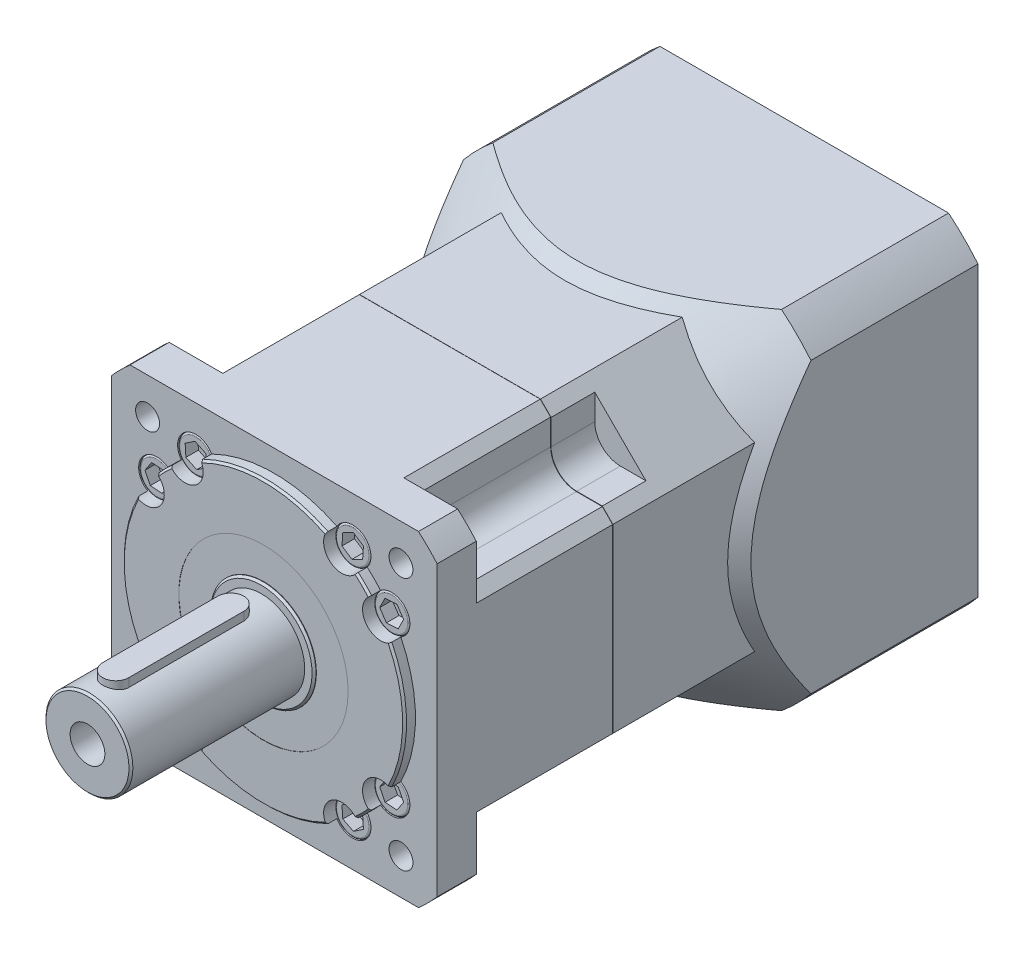
from build123d import *
from build123d.topology import SkipClean

# Parameters (mm, degrees)
EXTRUDE_START                    = 8
EXTRUDE_2_DEPTH                  = 15
CHAMFER_1_SIZE                   = 0.9
EXTRUDE_START_2                  = 49.5
SKETCH_6_W                       = 150
SKETCH_6_H                       = 150
EXTRUDE_1_DEPTH                  = 194.5
SKETCH_7_R                       = 5.5
CUT_EXTRUDE_1_DEPTH              = 18
CUT_EXTRUDE_START                = 226
CUT_EXTRUDE_3_DEPTH              = 176.5
CUT_EXTRUDE_2_DEPTH              = 83
CUT_EXTRUDE_4_DEPTH              = 62.8
PATTERN_CIRCULAR_1_COUNT         = 4
SKETCH_11_R                      = 8.4
CUT_EXTRUDE_5_DEPTH              = 5
CUT_EXTRUDE_START_2              = 244
SKETCH_12_R                      = 8.4
SKETCH_12_R_2                    = 8.25
CUT_EXTRUDE_6_DEPTH              = 9.9
CUT_EXTRUDE_7_DEPTH              = 5.775
FILLET_1_R                       = 0.825
PATTERN_CIRCULAR_2_COUNT         = 16
FILLET_1_OF_PATTERN_CIRCULAR_2_R = 0.825
CUT_EXTRUDE_START_3              = 248.9
SKETCH_14_R                      = 39
SKETCH_14_R_2                    = 24.3
CUT_EXTRUDE_8_DEPTH              = 0.1
EXTRUDE_3_DEPTH                  = 49.5
SKETCH_17_R                      = 4
CUT_EXTRUDE_9_DEPTH              = 24
PATTERN_CIRCULAR_3_COUNT         = 4
SKETCH_27_R                      = 150
CUT_EXTRUDE_15_DEPTH             = 143
SKETCH_21_R                      = 6.15
CUT_EXTRUDE_10_DEPTH             = 10
CUT_EXTRUDE_START_4              = 10
SKETCH_22_R                      = 6.15
SKETCH_22_R_2                    = 6
CUT_EXTRUDE_12_DEPTH             = 7.2
CUT_EXTRUDE_13_DEPTH             = 4.2
FILLET_2_R                       = 0.6
PATTERN_CIRCULAR_4_COUNT         = 4
FILLET_2_OF_PATTERN_CIRCULAR_4_R = 0.6
EXTRUDE_START_3                  = 10
EXTRUDE_4_DEPTH                  = 1
SKETCH_25_W                      = 150
SKETCH_25_H                      = 0.1
CUT_EXTRUDE_14_DEPTH             = 150


with BuildPart() as part:
    # 草图4 → 旋转1 (revolve)
    with BuildSketch(Plane(origin=(0, 0, 0), x_dir=(0, 0, -1), z_dir=(1, 0, 0))):
        Polygon((-249, 65), (-244, 65), (-244, 0), (-305.381197846, 0), (-310, 8), (-330, 8), (-330, 20), (-250, 20), (-250, 24.3), (-249, 24.3), align=None)
    revolve(axis=Axis((0, 0, 244), (0, 0, 1)))

    # 草图15 → 凸台-拉伸2 (add)
    with BuildSketch(Plane(origin=(0, 0, 0), x_dir=(1, 0, 0), z_dir=(0, 1, 0)).offset(EXTRUDE_START)):
        with BuildLine():
            Line((-6, -317), (-6, -264))
            ThreePointArc((-6, -264), (0, -258), (6, -264))
            Line((6, -264), (6, -317))
            ThreePointArc((6, -317), (0, -323), (-6, -317))
        make_face()
    extrude(amount=EXTRUDE_2_DEPTH)

    # 倒角1
    chamfer_1_edges = [part.edges().sort_by_distance(p)[0] for p in [
        (0, -65, 249),
        (0, -24.3, 250),
        (0, -20, 330),
    ]]
    chamfer(chamfer_1_edges, length=CHAMFER_1_SIZE)

    # 草图6 → 凸台-拉伸1 (add)
    with BuildSketch(Plane.XY.offset(EXTRUDE_START_2)):
        Rectangle(SKETCH_6_W, SKETCH_6_H)
    extrude(amount=EXTRUDE_1_DEPTH)

    # 草图7 → 切除-拉伸1 (cut)
    with BuildSketch(Plane.XY.offset(244)):
        with Locations((58.336309448, 58.336309448)):
            Circle(SKETCH_7_R)
        with BuildLine():
            Line((66.40732664, 75), (75, 75))
            Line((75, 75), (75, 66.40732664))
            ThreePointArc((75, 66.40732664), (70.834077362, 70.834077362), (66.40732664, 75))
        make_face()
    cut_extrude_1 = extrude(amount=-CUT_EXTRUDE_1_DEPTH, mode=Mode.SUBTRACT)

    # 草图9 → 切除-拉伸3 (cut)
    with BuildSketch(Plane.XY.offset(CUT_EXTRUDE_START)):
        Polygon((41.672618896, 75), (75, 41.672618896), (75, 75), align=None)
    cut_extrude_3 = extrude(amount=-CUT_EXTRUDE_3_DEPTH, mode=Mode.SUBTRACT)

    # 草图8 → 切除-拉伸2 (cut)
    with BuildSketch(Plane.XY.offset(CUT_EXTRUDE_START)):
        with BuildLine():
            Line((58.336309448, 46.553300859), (75, 46.553300859))
            Line((75, 46.553300859), (75, 75))
            Line((75, 75), (46.553300859, 75))
            Line((46.553300859, 75), (46.553300859, 58.336309448))
            ThreePointArc((46.553300859, 58.336309448), (50.004464172, 50.004464172), (58.336309448, 46.553300859))
        make_face()
    cut_extrude_2 = extrude(amount=-CUT_EXTRUDE_2_DEPTH, mode=Mode.SUBTRACT)

    # 草图10 → 切除-拉伸4 (cut)
    with BuildSketch(Plane(origin=(0, 0, 226), x_dir=(-1, 0, 0), z_dir=(0, 0, -1))):
        with BuildLine():
            Line((-46.553300859, 70.119318037), (-46.553300859, 58.336309448))
            ThreePointArc((-46.553300859, 58.336309448), (-50.004464172, 50.004464172), (-58.336309448, 46.553300859))
            Line((-58.336309448, 46.553300859), (-70.119318037, 46.553300859))
            Line((-70.119318037, 46.553300859), (-70.219318037, 46.453300859))
            Line((-70.219318037, 46.453300859), (-58.336309448, 46.453300859))
            ThreePointArc((-58.336309448, 46.453300859), (-49.933753494, 49.933753494), (-46.453300859, 58.336309448))
            Line((-46.453300859, 58.336309448), (-46.453300859, 70.219318037))
            Line((-46.453300859, 70.219318037), (-46.553300859, 70.119318037))
        make_face()
    cut_extrude_4 = extrude(amount=CUT_EXTRUDE_4_DEPTH, mode=Mode.SUBTRACT)

    # 阵列(圆周)1: 切除-拉伸1, 切除-拉伸3, 切除-拉伸2, 切除-拉伸4 ×4 about axis
    pattern_circular_1_axis = Axis((0, 0, 0), (0, 0, 1))
    add([cut_extrude_1.rotate(pattern_circular_1_axis, i * 360 / PATTERN_CIRCULAR_1_COUNT) for i in range(1, PATTERN_CIRCULAR_1_COUNT)], mode=Mode.SUBTRACT)
    add([cut_extrude_3.rotate(pattern_circular_1_axis, i * 360 / PATTERN_CIRCULAR_1_COUNT) for i in range(1, PATTERN_CIRCULAR_1_COUNT)], mode=Mode.SUBTRACT)
    add([cut_extrude_2.rotate(pattern_circular_1_axis, i * 360 / PATTERN_CIRCULAR_1_COUNT) for i in range(1, PATTERN_CIRCULAR_1_COUNT)], mode=Mode.SUBTRACT)
    add([cut_extrude_4.rotate(pattern_circular_1_axis, i * 360 / PATTERN_CIRCULAR_1_COUNT) for i in range(1, PATTERN_CIRCULAR_1_COUNT)], mode=Mode.SUBTRACT)

    # 草图11 → 切除-拉伸5 (cut)
    with BuildSketch(Plane.XY.offset(249)):
        with Locations((36.112065146, 54.0455248)):
            Circle(SKETCH_11_R)
    cut_extrude_5 = extrude(amount=-CUT_EXTRUDE_5_DEPTH, mode=Mode.SUBTRACT)

    # 草图12 → 切除-拉伸6 (cut)
    with BuildSketch(Plane.XY.offset(CUT_EXTRUDE_START_2)):
        with Locations((36.112065146, 54.0455248)):
            Circle(SKETCH_12_R)
        with Locations((36.112065146, 54.0455248)):
            Circle(SKETCH_12_R_2, mode=Mode.SUBTRACT)
    cut_extrude_6 = extrude(amount=-CUT_EXTRUDE_6_DEPTH, mode=Mode.SUBTRACT)

    # 草图13 → 切除-拉伸7 (cut)
    with BuildSketch(Plane.XY.offset(CUT_EXTRUDE_START_2)):
        Polygon((40.685148014, 50.989888518), (41.044865225, 56.478112596), (36.471782357, 59.533748877), (31.538982279, 57.101161081), (31.179265068, 51.612937003), (35.752347936, 48.557300722), align=None)
    cut_extrude_7 = extrude(amount=-CUT_EXTRUDE_7_DEPTH, mode=Mode.SUBTRACT)

    # 圆角1
    fillet_1_edges = [part.edges().sort_by_distance(p)[0] for p in [
        (27.862065146, 54.0455248, 244),
    ]]
    fillet(fillet_1_edges, radius=FILLET_1_R)

    # 阵列(圆周)2: 切除-拉伸5, 切除-拉伸6, 切除-拉伸7 ×16 about axis, 8 skipped
    pattern_circular_2_axis = Axis((0, 0, 0), (0, 0, -1))
    add([cut_extrude_5.rotate(pattern_circular_2_axis, i * 360 / PATTERN_CIRCULAR_2_COUNT) for i in range(1, PATTERN_CIRCULAR_2_COUNT) if i not in (2, 3, 6, 7, 10, 11, 14, 15)], mode=Mode.SUBTRACT)
    add([cut_extrude_6.rotate(pattern_circular_2_axis, i * 360 / PATTERN_CIRCULAR_2_COUNT) for i in range(1, PATTERN_CIRCULAR_2_COUNT) if i not in (2, 3, 6, 7, 10, 11, 14, 15)], mode=Mode.SUBTRACT)
    add([cut_extrude_7.rotate(pattern_circular_2_axis, i * 360 / PATTERN_CIRCULAR_2_COUNT) for i in range(1, PATTERN_CIRCULAR_2_COUNT) if i not in (2, 3, 6, 7, 10, 11, 14, 15)], mode=Mode.SUBTRACT)

    # 圆角1 of 阵列(圆周)2
    fillet_1_of_pattern_circular_2_edges = [part.edges().sort_by_distance(p)[0] for p in [
        (46.423518656, 39.269203463, 244),
        (54.0455248, -27.862065146, 244),
        (39.269203463, -46.423518656, 244),
        (-27.862065146, -54.0455248, 244),
        (-46.423518656, -39.269203463, 244),
        (-54.0455248, 27.862065146, 244),
        (-39.269203463, 46.423518656, 244),
    ]]
    fillet(fillet_1_of_pattern_circular_2_edges, radius=FILLET_1_OF_PATTERN_CIRCULAR_2_R)

    # 草图14 → 切除-拉伸8 (cut)
    with BuildSketch(Plane.XY.offset(CUT_EXTRUDE_START_3)):
        Circle(SKETCH_14_R)
        with Locations(Location((0, 0, 0), (0, 0, 90))):
            Circle(SKETCH_14_R_2, mode=Mode.SUBTRACT)
    extrude(amount=CUT_EXTRUDE_8_DEPTH, mode=Mode.SUBTRACT)

    # 草图16 → 凸台-拉伸3 (add)
    with BuildSketch(Plane.XY):
        with BuildLine():
            Line((80, -66.452990903), (80, 66.452990903))
            ThreePointArc((80, 66.452990903), (73.539105243, 73.539105243), (66.452990903, 80))
            Line((66.452990903, 80), (-66.452990903, 80))
            ThreePointArc((-66.452990903, 80), (-73.539105243, 73.539105243), (-80, 66.452990903))
            Line((-80, 66.452990903), (-80, -66.452990903))
            ThreePointArc((-80, -66.452990903), (-73.539105243, -73.539105243), (-66.452990903, -80))
            Line((-66.452990903, -80), (66.452990903, -80))
            ThreePointArc((66.452990903, -80), (73.539105243, -73.539105243), (80, -66.452990903))
        make_face()
    extrude(amount=EXTRUDE_3_DEPTH)

    # 草图17 → 切除-拉伸9 (cut)
    with BuildSketch(Plane.XY):
        with Locations((51.265241636, 51.265241636)):
            Circle(SKETCH_17_R)
    cut_extrude_9 = extrude(amount=CUT_EXTRUDE_9_DEPTH, mode=Mode.SUBTRACT)

    # 阵列(圆周)3: 切除-拉伸9 ×4 about axis
    pattern_circular_3_axis = Axis((0, 0, 0), (0, 0, 1))
    for i in range(1, PATTERN_CIRCULAR_3_COUNT):
        add(cut_extrude_9.rotate(pattern_circular_3_axis, i * 360 / PATTERN_CIRCULAR_3_COUNT), mode=Mode.SUBTRACT)

    # 草图26 → 旋转2 (revolve)
    with BuildSketch(Plane(origin=(0, 0, 0), x_dir=(0, 0, -1), z_dir=(1, 0, 0)), mode=Mode.PRIVATE) as revolve_2_sk:
        Polygon((-24, 150), (-24, 0), (-196.552629984, 0), align=None)
    revolve(revolve_2_sk.sketch.rotate(Axis((0, 0, 196.552629984), (0, 0, -1)), 180), axis=Axis((0, 0, 196.552629984), (0, 0, -1)))

    # 草图27 → 切除-拉伸15 (cut)
    with BuildSketch(Plane(origin=(0, 0, 0), x_dir=(-1, 0, 0), z_dir=(0, 0, -1))):
        Circle(SKETCH_27_R)
        with BuildLine():
            Line((-66.452990903, 80), (66.452990903, 80))
            ThreePointArc((66.452990903, 80), (73.539105243, 73.539105243), (80, 66.452990903))
            Line((80, 66.452990903), (80, -66.452990903))
            ThreePointArc((80, -66.452990903), (73.539105243, -73.539105243), (66.452990903, -80))
            Line((66.452990903, -80), (-66.452990903, -80))
            ThreePointArc((-66.452990903, -80), (-73.539105243, -73.539105243), (-80, -66.452990903))
            Line((-80, -66.452990903), (-80, 66.452990903))
            ThreePointArc((-80, 66.452990903), (-73.539105243, 73.539105243), (-66.452990903, 80))
        make_face(mode=Mode.SUBTRACT)
    extrude(amount=-CUT_EXTRUDE_15_DEPTH, mode=Mode.SUBTRACT)

    # 草图20 → 切除-旋转1 (revolve, cut)
    with BuildSketch(Plane(origin=(0, 0, 0), x_dir=(0, 0, -1), z_dir=(1, 0, 0)), mode=Mode.PRIVATE) as cut_revolve_1_sk:
        Polygon((0, 55), (-10, 55), (-10, 11), (-62, 11), (-62, 0), (0, 0), align=None)
    revolve(cut_revolve_1_sk.sketch.rotate(Axis((0, 0, 0), (0, 0, 1)), 119.058078704), axis=Axis((0, 0, 0), (0, 0, 1)), mode=Mode.SUBTRACT)

    # 草图21 → 切除-拉伸10 (cut)
    with BuildSketch(Plane.XY):
        with Locations((-21.04758878, 50.813374288)):
            Circle(SKETCH_21_R)
    cut_extrude_10 = extrude(amount=CUT_EXTRUDE_10_DEPTH, mode=Mode.SUBTRACT)

    # 草图22 → 切除-拉伸12 (cut)
    with BuildSketch(Plane.XY.offset(CUT_EXTRUDE_START_4)):
        with Locations(Location((-21.04758878, 50.813374288, 0), (0, 0, 205.705026153))):
            Circle(SKETCH_22_R)
        with Locations((-21.04758878, 50.813374288)):
            Circle(SKETCH_22_R_2, mode=Mode.SUBTRACT)
    cut_extrude_12 = extrude(amount=CUT_EXTRUDE_12_DEPTH, mode=Mode.SUBTRACT)

    # 草图23 → 切除-拉伸13 (cut)
    with BuildSketch(Plane.XY.offset(CUT_EXTRUDE_START_4)):
        Polygon((-20.525484011, 54.779153734), (-24.221002141, 53.248420004), (-24.74310691, 49.282640559), (-21.569693549, 46.847594843), (-17.874175419, 48.378328572), (-17.35207065, 52.344108018), align=None)
    cut_extrude_13 = extrude(amount=CUT_EXTRUDE_13_DEPTH, mode=Mode.SUBTRACT)

    # 圆角2
    fillet_2_edges = [part.edges().sort_by_distance(p)[0] for p in [
        (-27.04758878, 50.813374288, 10),
    ]]
    fillet(fillet_2_edges, radius=FILLET_2_R)

    # 阵列(圆周)4: 切除-拉伸10, 切除-拉伸12, 切除-拉伸13 ×4 about axis
    pattern_circular_4_axis = Axis((0, 0, 0), (0, 0, 1))
    add([cut_extrude_10.rotate(pattern_circular_4_axis, i * 360 / PATTERN_CIRCULAR_4_COUNT) for i in range(1, PATTERN_CIRCULAR_4_COUNT)], mode=Mode.SUBTRACT)
    add([cut_extrude_12.rotate(pattern_circular_4_axis, i * 360 / PATTERN_CIRCULAR_4_COUNT) for i in range(1, PATTERN_CIRCULAR_4_COUNT)], mode=Mode.SUBTRACT)
    add([cut_extrude_13.rotate(pattern_circular_4_axis, i * 360 / PATTERN_CIRCULAR_4_COUNT) for i in range(1, PATTERN_CIRCULAR_4_COUNT)], mode=Mode.SUBTRACT)

    # 圆角2 of 阵列(圆周)4
    fillet_2_of_pattern_circular_4_edges = [part.edges().sort_by_distance(p)[0] for p in [
        (-50.813374288, -27.04758878, 10),
        (27.04758878, -50.813374288, 10),
        (50.813374288, 27.04758878, 10),
    ]]
    fillet(fillet_2_of_pattern_circular_4_edges, radius=FILLET_2_OF_PATTERN_CIRCULAR_4_R)

    # 草图24 → 凸台-拉伸4 (add)
    with SkipClean():  # the faces are left unmerged after this step: merging them gives an invalid solid
        with BuildSketch(Plane.XY.offset(EXTRUDE_START_3)):
            with BuildLine():
                Line((0.25, 32.999053017), (0.25, 10.997158724))
                ThreePointArc((0.25, 10.997158724), (11, 0), (0.25, -10.997158724))
                Line((0.25, -10.997158724), (0.25, -32.999053017))
                ThreePointArc((0.25, -32.999053017), (33, 0), (0.25, 32.999053017))
            make_face()
            with BuildLine():
                Line((-0.25, 32.999053017), (-0.25, 10.997158724))
                ThreePointArc((-0.25, 10.997158724), (-11, 0), (-0.25, -10.997158724))
                Line((-0.25, -10.997158724), (-0.25, -32.999053017))
                ThreePointArc((-0.25, -32.999053017), (-33, 0), (-0.25, 32.999053017))
            make_face()
        extrude(amount=-EXTRUDE_4_DEPTH)

    # 草图25 → 切除-拉伸14 (cut)
    with SkipClean():  # the faces are left unmerged after this step: merging them gives an invalid solid
        with BuildSketch(Plane(origin=(0, 75, 0), x_dir=(1, 0, 0), z_dir=(0, 1, 0))):
            with Locations((0, -163.15)):
                Rectangle(SKETCH_25_W, SKETCH_25_H)
        extrude(amount=-CUT_EXTRUDE_14_DEPTH, mode=Mode.SUBTRACT)


with BuildPart() as cut_extrude_14_piece_1:
    # of the separate pieces the step leaves, piece 1, a body of its own (cut_extrude_14_pieces)
    add(part.part.solids().sort_by_distance((-50.813374288, -15.04758878, 10.6))[0])


with BuildPart() as cut_extrude_14_piece_2:
    # of the separate pieces the step leaves, piece 2, a body of its own (cut_extrude_14_pieces)
    add(part.part.solids().sort_by_distance((-41.672618896, -75, 163.2))[0])


solid = Compound([cut_extrude_14_piece_1.part, cut_extrude_14_piece_2.part])
